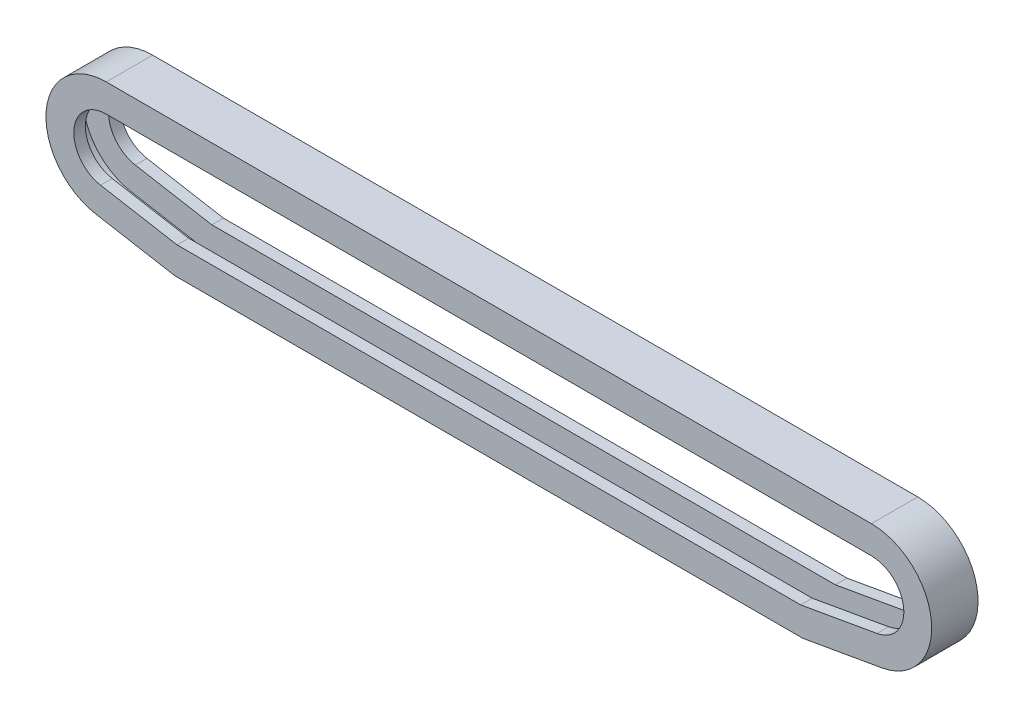
SolidWorks part; units mm, degrees
ref_plane "Front Plane" through (0, 0, 0) normal (0, 0, 1) x (1, 0, 0)
ref_plane "Top Plane" through (0, 0, 0) normal (0, 1, 0) x (1, 0, 0)
ref_plane "Right Plane" through (0, 0, 0) normal (1, 0, 0) x (0, 0, -1)
sketch "Sketch2" plane through (0, 0, 0) normal (0, 0, 1) x (1, 0, 0)
  line L0 (165, 0) -> (-165, 0) construction
  line L1 (0, 0) -> (0, -25.5983) construction
  line L2 (-135, -25.5983) -> (-168.473, -19.6962) construction
  line L3 (135, -25.5983) -> (168.473, -19.6962) construction
  line L4 (-165, 20) -> (165, 20) construction
  line L5 (-135, -25.5983) -> (135, -25.5983) construction
  line L6 (-165, 0) -> (-168.473, -19.6962) construction
  line L7 (-165, 26) -> (165, 26)
  line L8 (135.5249, -31.5983) -> (169.5149, -25.605)
  line L9 (-135.5249, -31.5983) -> (135.5249, -31.5983)
  line L10 (-135.5249, -31.5983) -> (-169.5149, -25.605)
  line L11 (-165, 14) -> (165, 14)
  line L12 (134.4751, -19.5983) -> (167.4311, -13.7873)
  line L13 (-134.4751, -19.5983) -> (134.4751, -19.5983)
  line L14 (-134.4751, -19.5983) -> (-167.4311, -13.7873)
  arc A0 (-165, 20) -> (-168.473, -19.6962) centre (-165, 0) ccw construction
  arc A1 (165, 20) -> (168.473, -19.6962) centre (165, 0) cw construction
  arc A2 (165, 26) -> (169.5149, -25.605) centre (165, 0) cw
  arc A3 (-165, 26) -> (-169.5149, -25.605) centre (-165, 0) ccw
  arc A4 (165, 14) -> (167.4311, -13.7873) centre (165, 0) cw
  arc A5 (-165, 14) -> (-167.4311, -13.7873) centre (-165, 0) ccw
  point P6 (0, 0)
  dimension "D1" = 40
  dimension "D7" = 26
  dimension "D8" = 14
  dimension "D2" = 330
  dimension "D3" = 30
  dimension "D4" = 100
  dimension "D5" = 6
  dimension "D6" = 6
extrude "Boss-Extrude1" add sketch "Sketch2" along normal mid plane 20
sketch "Sketch8" plane through (0, 0, 0) normal (0, 0, 1) x (1, 0, 0)
  line L18 (135.4374, -30.5983) -> (169.3412, -24.6202)
  line L19 (-135.4374, -30.5983) -> (135.4374, -30.5983)
  line L20 (-169.3412, -24.6202) -> (-135.4374, -30.5983)
  line L21 (165, 25) -> (-165, 25)
  line L22 (135.4374, -30.5983) -> (169.3412, -24.6202)
  line L23 (-135.4374, -30.5983) -> (135.4374, -30.5983)
  line L24 (-169.3412, -24.6202) -> (-135.4374, -30.5983)
  line L25 (165, 25) -> (-165, 25)
  arc A12 (169.3412, -24.6202) -> (165, 25) centre (165, 0) ccw
  arc A13 (-165, 25) -> (-169.3412, -24.6202) centre (-165, 0) ccw
  arc A14 (169.3412, -24.6202) -> (165, 25) centre (165, 0) ccw
  arc A15 (-165, 25) -> (-169.3412, -24.6202) centre (-165, 0) ccw
  dimension "D1" = 1
extrude "Cut-Extrude1" cut sketch "Sketch8" against normal mid plane 10
